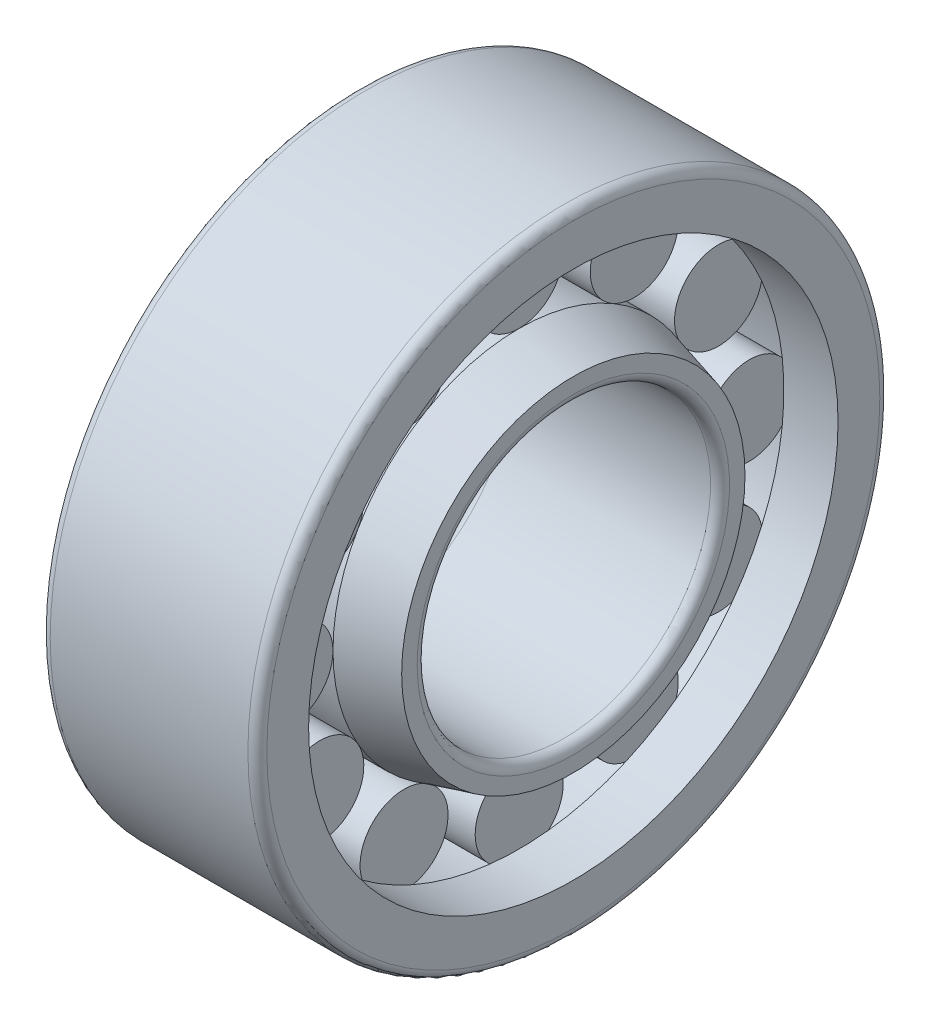
from build123d import *

# Parameters (mm, degrees)
SKETCH3_W         = 24
SKETCH3_H         = 9.7501
CIRPATTERN1_COUNT = 12


with BuildPart() as part:
    # Sketch2 → Base-Revolve (revolve)
    with BuildSketch(Plane.XY, mode=Mode.PRIVATE) as base_revolve_sk:
        with BuildLine():
            Line((36, 41.25), (12, 41.25))
            Line((12, 41.25), (0.002884361, 34.489972754))
            ThreePointArc((0.002884361, 34.489972754), (0.654499605, 33.076671865), (2.1, 32.5))
            Line((2.1, 32.5), (45.9, 32.5))
            ThreePointArc((45.9, 32.5), (47.38492424, 33.11507576), (48, 34.6))
            Line((48, 34.6), (48, 38.034609691))
            Line((48, 38.034609691), (36, 41.25))
        make_face()
    revolve(base_revolve_sk.sketch.rotate(Axis((-10.080094127, 0, 0), (1, 0, 0)), 90), axis=Axis((-10.080094127, 0, 0), (1, 0, 0)))

    # Sketch3 → Boss-Revolve1 (revolve)
    with BuildSketch(Plane.XY):
        with Locations((24, 46.12495)):
            Rectangle(SKETCH3_W, SKETCH3_H)
    boss_revolve1 = revolve(axis=Axis((-1.603948851, 51, 0), (1, 0, 0)))

    # Sketch4 → Boss-Revolve2 (revolve)
    with BuildSketch(Plane.XY, mode=Mode.PRIVATE) as boss_revolve2_sk:
        with BuildLine():
            Line((36, 58.65), (48, 58.65))
            Line((48, 58.65), (48, 67.9))
            ThreePointArc((48, 67.9), (47.38492424, 69.38492424), (45.9, 70))
            Line((45.9, 70), (2.1, 70))
            ThreePointArc((2.1, 70), (0.61507576, 69.38492424), (0, 67.9))
            Line((0, 67.9), (0, 58.65))
            Line((0, 58.65), (12, 58.65))
            Line((12, 58.65), (12, 60.75))
            Line((12, 60.75), (36, 60.75))
            Line((36, 60.75), (36, 58.65))
        make_face()
    revolve(boss_revolve2_sk.sketch.rotate(Axis((0, 0, 0), (1, 0, 0)), 90), axis=Axis((0, 0, 0), (1, 0, 0)))

    # CirPattern1: Boss-Revolve1 ×12 about axis
    cirpattern1_axis = Axis((0, 0, 0), (1, 0, 0))
    for i in range(1, CIRPATTERN1_COUNT):
        add(boss_revolve1.rotate(cirpattern1_axis, i * 360 / CIRPATTERN1_COUNT))


solid = part.part
